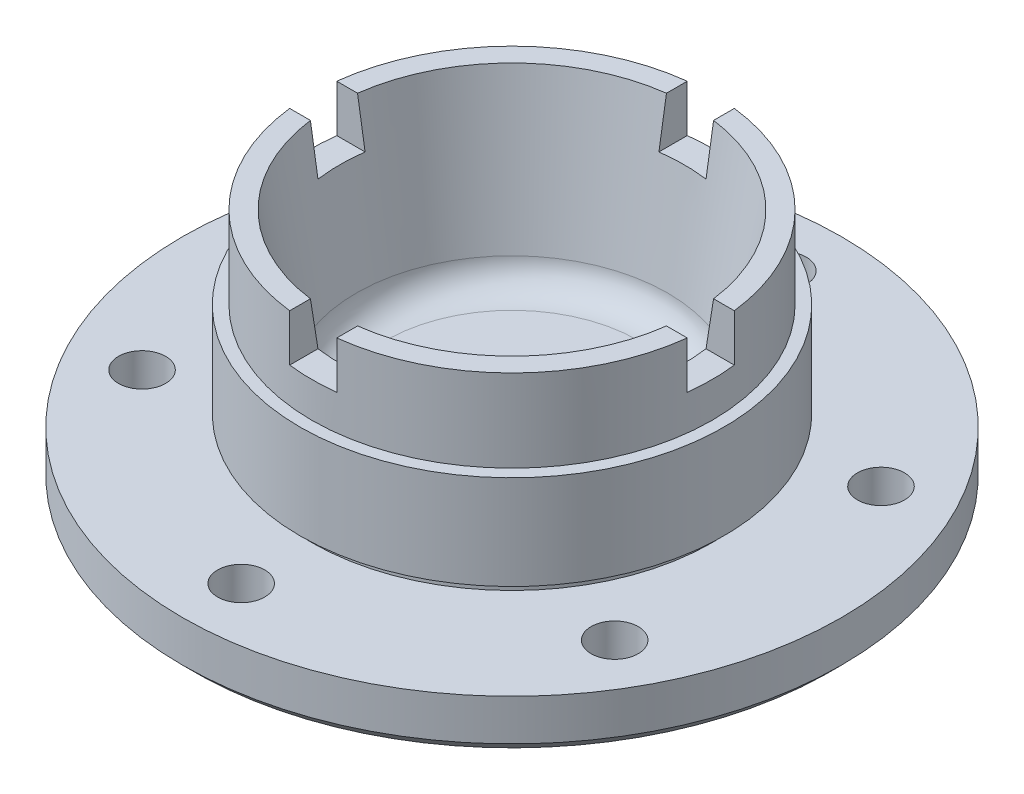
from build123d import *

# Parameters (mm, degrees)
SKETCH2_W          = 20
SKETCH2_H          = 8
SKETCH2_W_2        = 8
SKETCH2_H_2        = 20
CUT_EXTRUDE1_DEPTH = 8
SKETCH3_R          = 4
CUT_EXTRUDE2_DEPTH = 100
SCALE_1_SCALE      = 1.875


with BuildPart() as part:
    # Sketch1 → Revolve1 (revolve)
    with BuildSketch(Plane.XY, mode=Mode.PRIVATE) as revolve1_sk:
        with BuildLine():
            Line((32, 0), (54, 0))
            Line((54, 0), (56, 2))
            Line((56, 2), (56, 9))
            Line((56, 9), (36, 9))
            Line((36, 9), (34, 9))
            Line((34, 9), (34, 11))
            Line((34, 11), (36, 11))
            Line((36, 11), (36, 27))
            Line((36, 27), (34, 27))
            Line((34, 27), (34, 41))
            Line((34, 41), (30.5, 41))
            Line((30.5, 41), (26.45024814, 15.502481405))
            ThreePointArc((26.45024814, 15.502481405), (24.830088793, 12.292737332), (21.475062189, 11))
            Line((21.475062189, 11), (0, 11))
            Line((0, 11), (0, 2))
            Line((0, 2), (31, 2))
            Line((31, 2), (32, 0))
        make_face()
    revolve(revolve1_sk.sketch.rotate(Axis((0, 2, 0), (0, 1, 0)), 90), axis=Axis((0, 2, 0), (0, 1, 0)))

    # Sketch2 → Cut-Extrude1 (cut)
    with BuildSketch(Plane(origin=(0, 41, 0), x_dir=(1, 0, 0), z_dir=(0, 1, 0))):
        with Locations((27.262332301, 0)):
            Rectangle(SKETCH2_W, SKETCH2_H)
        with Locations((0, 27.262332301)):
            Rectangle(SKETCH2_W_2, SKETCH2_H_2)
        with Locations((0, -27.262332301)):
            Rectangle(SKETCH2_W_2, SKETCH2_H_2)
        with Locations((-27.262332301, 0)):
            Rectangle(SKETCH2_W, SKETCH2_H)
    extrude(amount=-CUT_EXTRUDE1_DEPTH, mode=Mode.SUBTRACT)

    # Sketch3 → Cut-Extrude2 (cut)
    with BuildSketch(Plane(origin=(0, 41, 0), x_dir=(1, 0, 0), z_dir=(0, 1, 0))):
        with Locations(Location((0, 46, 0), (0, 0, 270))):
            Circle(SKETCH3_R)
        with Locations(Location((40.056631801, 22.615619575, 0), (0, 0, 270))):
            Circle(SKETCH3_R)
        with Locations(Location((-39.837168574, 23, 0), (0, 0, 270))):
            Circle(SKETCH3_R)
        with Locations(Location((-39.837168574, -23, 0), (0, 0, 270))):
            Circle(SKETCH3_R)
        with Locations(Location((0, -46, 0), (0, 0, 270))):
            Circle(SKETCH3_R)
        with Locations(Location((40.056631801, -22.615619575, 0), (0, 0, 270))):
            Circle(SKETCH3_R)
    extrude(amount=-CUT_EXTRUDE2_DEPTH, mode=Mode.SUBTRACT)


with BuildPart() as part_1:
    # Scale 1: scaled about (-0.001562363, 10.8729077, 0)
    add(part.part.scale(SCALE_1_SCALE).moved(Location((0.001367068, -9.513794238, 0))))


solid = part_1.part
